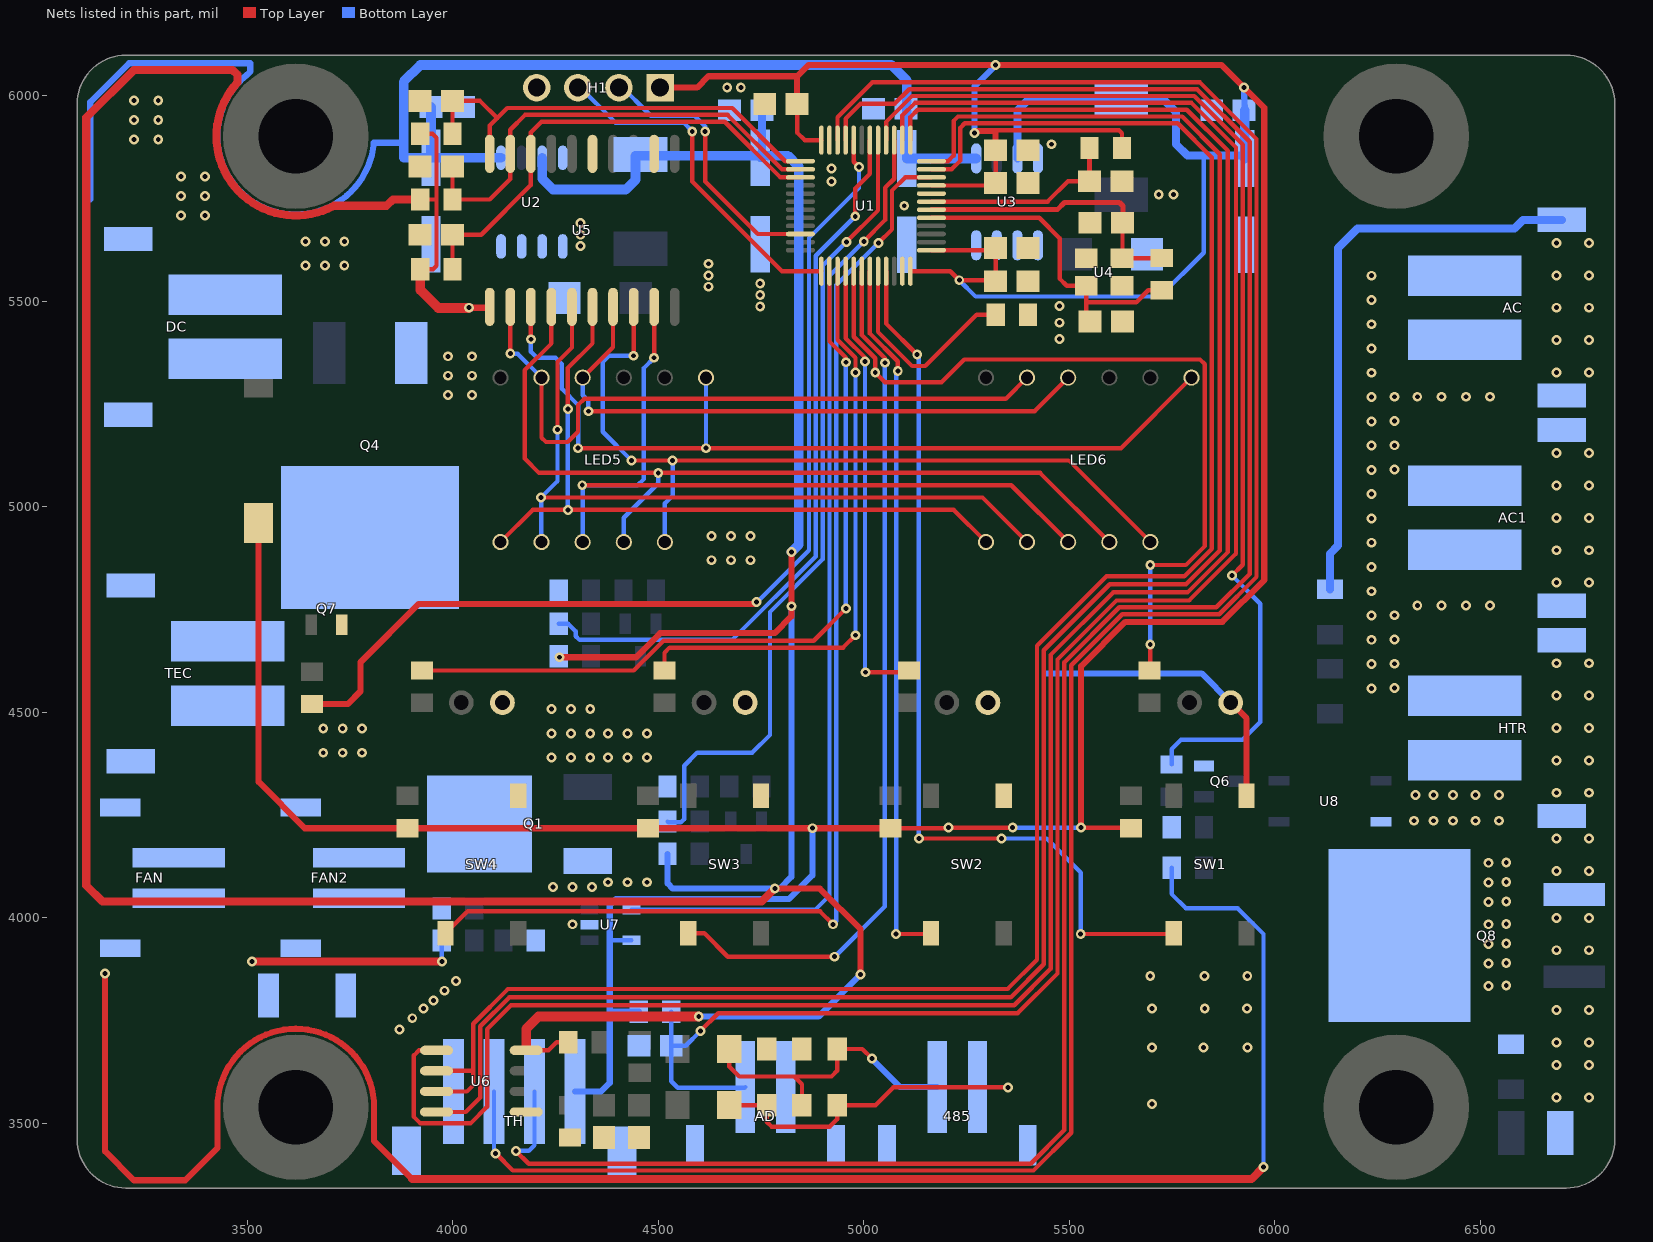
[diagram p0: the nets of this part, all layers, seen from the top]
# Altium PCB MISC82750.pcbdoc (part 2 of 3)
Units mil, origin at the board's own origin, x right, y up, seen from the top; angles counter-clockwise.
Board outline 3740.2 x 2755.9 mil, 2 copper layers (Top Layer, Bottom Layer), stack 62.2 mil thick; 106 components, 84 nets, 362 pads, 334 vias.

## Via types
v1: diameter 24, hole 12, Top Layer to Bottom Layer, 334 vias

## Nets (pads, with @x,y where several pads share a name; then routed paths per layer and width w, separated by ;. In a path a pad name is that pad's centre, name@x,y a point inside that pad or via, vN(x,y) a via of type N, cw(c..) or ccw(c..) an arc to the next point about the centre after c; other vN are vias at no path point) (continued)
+3.3V: BUZZER1.1 C7.2 C8.1 C11.2 C12.2 C13.2 C14.2 C20.2 H1.1 L2.1 R3.2 R7.2 R12.2 R13.2 R14.2 R15.2 TH.1 U1.1 U1.9 U1.24 U1.48 U3.3 U7.5 | length 11081.4
  Top Layer w10.6: C11.2@4837.7,5980 4837.7,5910.3 4856.1,5892 U1.24@4896.8,5892 ; R13.2@5065,4218.1 5204.5,4218.1 v1(5205.8,4219.4) v1(5362.2,4219.4) ; U1.48@5113.3,5573.1 5210.4,5573.1 v1(5232.3,5551.2) 5318.2,5551.2 C13.2@5320.7,5548.7 C14.2@5320.7,5629.4 5315.5,5624.2 U1.1@5164.5,5624.2 ; U1.9@5164.5,5781.7 5314.9,5781.7 C12.2@5320.7,5787.5 C20.2@5320.7,5867.5 ; 5320.7,5913.8 5320.7,5916.1 5620.9,5916.1 5628,5909 R3.2@5628,5873.1 ; v1(5528.5,4219.4) 5648.8,4219.4 R12.2@5650,4218.1
  Top Layer w15: BUZZER1.1@3527.6,4960.6 3527.6,4330.7 3640.1,4218.1 R15.2@3890,4218.1 R14.2@4475,4218.1 v1(4875.1,4218.1) R13.2@5065,4218.1 ; H1.1@4504.3,6019.7 4594.5,6019.7 4622,6047.2 4837.7,6047.2 ; C11.2@4837.7,5980 4837.7,6047.2 ; v1(5269.5,5909.4) 5274,5914 5320.5,5914 5320.7,5913.8 C20.2@5320.7,5867.5 ; v1(5528.5,4219.4) 5528.5,4612.1 5636.3,4720 5872.4,4720 5974.2,4821.7 5974.2,5970.7 v1(5925.2,6019.7) 5870.3,6074.6 v1(5320.7,6074.6) 4865.1,6074.6 4837.7,6047.2
  Bottom Layer w10.6: 4381.9,3945.6 U7.5@4434.9,3945.6 ; v1(5232.3,5551.2) 5272,5511.5 5720.2,5511.5 5826.8,5618.1 5826.8,5854.3 ; v1(5362.2,4219.4) v1(5528.5,4219.4)
  Bottom Layer w15: TH.1@4297.2,3577.6 4361,3577.6 4381.9,3598.4 4381.9,3771.7 ; R7.2@4452.8,3771.7 4381.9,3771.7 ; v1(4875.1,4218.1) 4875.1,4103.5 4817.3,4045.7 4396.9,4045.7 4381.9,4030.7 4381.9,3945.6 4381.9,3771.7 ; v1(5269.5,5909.4) 5269.5,6023.4 v1(5320.7,6074.6) ; v1(5925.2,6019.7) C7.2@5926.6,5964.6
  Bottom Layer w19.7: U3.3@5373.6,5847.4 5373.6,5964.1 5401.6,5992.1 5622.6,5992.1 L2.1@5626,5988.7 5731.8,5988.7 5759.8,5960.6 5759.8,5881.9 5787.4,5854.3 5826.8,5854.3 5919.6,5854.3 C8.1@5926.6,5847.4
  Bottom Layer w23.6: C8.1@5926.6,5847.4 C7.2@5926.6,5964.6
+5V: C3.2 C4.1 L1.1 R4.2 R5.2 R6.2 R20.1 R25.1 R35.2 U2.3 U5.1 U6.8 | length 10482.4
  Top Layer w10.6: R6.2@3920.7,5578.1 3952.1,5578.1 3960.6,5586.6 3960.6,5630.5 3960.4,5630.8 3960.4,5748.3 ; R5.2@3920.7,5747.5 3959.6,5747.5 3960.4,5748.3 ; R4.2@3920.7,5907.5 3950.7,5907.5 3960.6,5897.6 3960.6,5859.1 3960.4,5858.8 3960.4,5748.3 ; U6.8@4178.6,3677.7 4232.8,3677.7 4252.6,3697.5 R35.2@4280.7,3697.5
  Top Layer w15: v1(4039.4,5484.3) 4088,5484.3 U5.1@4090,5486.3 ; v1(4259.8,4633.9) 4445.9,4633.9 4504.9,4692.9 4783.5,4692.9 4824,4733.4 v1(4824,4758) v1(4824,4889.8) ; v1(4783.5,4071.1) 4893.4,4071.1 4992.1,3972.4 v1(4992.1,3862.2)
  Top Layer w19.7: 3475.81,6031.99 ccw(c3618.1,5901.6) 3425.1,5901.6 ccw(c3618.1,5901.6) 3710.78,5732.31 3838.6,5732.3 3854.3,5748 3920.2,5748 R5.2@3920.7,5747.5 ; 3475.9,6032 3475.9,6051.7 3464.6,6063 3224.4,6063 3108.3,5946.9 3108.3,4078.7 3147.6,4039.4 4751.7,4039.4 v1(4783.5,4071.1)
  Top Layer w23.6: R6.2@3920.7,5578.1 3921.3,5577.5 3921.3,5527.6 3965,5483.8 4039,5483.8 v1(4039.4,5484.3) ; U6.8@4178.6,3677.7 4178.6,3729.7 4208.7,3759.8 v1(4598.4,3759.8)
  Bottom Layer w10.6: R25.1@4257.6,4636.6 4257.6,4636.1 v1(4259.8,4633.9)
  Bottom Layer w15: R20.1@4522.6,4155.6 4522.6,4083.7 4535.2,4071.1 v1(4783.5,4071.1) 4795.5,4071.1 4824,4099.5 v1(4824,4758) ; v1(4598.4,3759.8) 4889.8,3759.8 v1(4992.1,3862.2)
  Bottom Layer w19.7: C4.1@4747.8,5849.1 4752,5853.3 4752,5854.3 C3.2@4752,5964.6
  Bottom Layer w23.6: U2.3@4217.6,5849.1 4217.6,5798.1 4244.1,5771.7 4420.9,5771.7 4444.5,5795.3 4444.5,5854.3 4752,5854.3 4815,5854.3 4841.6,5827.7 4841.6,4907.4 v1(4824,4889.8)
A: LED5.11 LED6.11 U5.2 | length 1648.6
  Top Layer w10.6: v1(4140,5372.5) U5.2@4140,5486.3 ; LED5.11@4216.1,5314.2 4216.1,5168.1 4226.8,5157.5 4280,5157.5 4304.8,5182.3 4304.8,5247.3 4320,5262.5 5345.6,5262.5 LED6.11@5397.2,5314.2
  Bottom Layer w10.6: v1(4140,5372.5) 4157.8,5372.5 LED5.11@4216.1,5314.2
AD: AD.1 C19.2 R7.1 U1.14 | length 4591.6
  Top Layer w10.6: v1(4602.4,3724.4) 4645.7,3767.7 5374.2,3767.7 5471.1,3864.6 5471.1,4628.4 5614.7,4772 5791.4,4772 5905.5,4886.1 5905.5,5874.2 5797.1,5982.6 5124.4,5982.6 5093.6,5951.9 U1.14@5093.6,5892
  Bottom Layer w10.6: R7.1@4531.5,3771.7 C19.2@4531.5,3689 ; v1(4602.4,3724.4) 4566.9,3689 C19.2@4531.5,3689 ; AD.1@4711.7,3588.4 4710,3586.6 4547.2,3586.6 4531.5,3602.4 C19.2@4531.5,3689
AD5: U1.15 U7.4 | length 2398.5
  Top Layer w10.6: v1(5000,5645.7) 5051.9,5697.6 5051.9,5776.2 5073.9,5798.2 U1.15@5073.9,5892
  Bottom Layer w10.6: U7.4@4434.9,4020.4 4882.6,4020.4 4916.4,4054.2 4916.4,5562.1 v1(5000,5645.7)
B: LED5.7 LED6.7 U5.3 | length 2152.8
  Top Layer w10.6: v1(4190,5407.5) U5.3@4190,5486.3 ; v1(4305,5142.5) v1(4616.1,5142.5) 5625.6,5142.5 LED6.7@5797.2,5314.2
  Bottom Layer w10.6: v1(4190,5407.5) 4190,5377.5 4205,5362.5 4250,5362.5 4265,5347.5 4265,5287.5 4305,5247.5 v1(4305,5142.5) ; v1(4616.1,5142.5) LED5.7@4616.1,5314.2
BOOT0: R2.2 U1.44 | length 519.9
  Top Layer w10.6: U1.44@5034.6,5573.1 5034.6,5425.4 5117.5,5342.5 5149.6,5342.5 5274.6,5467.5 R2.2@5320.7,5467.5
BUZZER: R38.1 U1.20 | length 2459
  Top Layer w10.6: U1.20@4975.5,5892 4975.5,5839.5 v1(4988.2,5826.8)
  Top Layer w15: R38.1@3657.5,4520.1 3744.5,4520.1 3775.6,4551.2 3775.6,4622 3917.3,4763.8 4734.8,4763.8 v1(4739.1,4768.1)
  Bottom Layer w10.6: v1(4739.1,4768.1) 4740.6,4768.1 4866.6,4894.1 4866.6,5654 4988.2,5775.6 v1(4988.2,5826.8)
C: LED5.4 LED6.4 U5.4 | length 2105.2
  Top Layer w10.6: U5.4@4240,5486.3 4240,5397.5 4175,5332.5 4175,5117.5 4210,5082.5 v1(4500,5082.5) 5428.9,5082.5 LED6.4@5597.2,4914.2
  Bottom Layer w10.6: LED5.4@4416.1,4914.2 4416.1,4973.6 4500,5057.5 v1(4500,5082.5)
CLK: C17.2 R5.1 U1.26 U5.19 | length 1136.5
  Top Layer w10.6: C17.2@3999.4,5827.5 R5.1@3999.4,5747.5 4090,5747.5 4140,5797.5 U5.19@4140,5858.7 4140,5917.5 4175.8,5953.3 4668.7,5953.3 4800.9,5821.1 U1.26@4845.6,5821.1
D: LED5.2 LED6.2 U5.5 | length 1830.7
  Top Layer w10.6: v1(4215,5022.5) 5288.9,5022.5 LED6.2@5397.2,4914.2 ; v1(4255,5187.5) 4255,5352.5 4290,5387.5 U5.5@4290,5486.3
  Bottom Layer w10.6: LED5.2@4216.1,4914.2 4215,4915.3 v1(4215,5022.5) 4255,5062.5 v1(4255,5187.5)
DIN: C18.2 R6.1 U1.27 U5.18 | length 1175
  Top Layer w10.6: R6.1@3999.4,5578.1 C18.2@3999.4,5662 4069.5,5662 4190,5782.5 U5.18@4190,5858.7 4190,5910.6 4216.1,5936.7 4661.8,5936.7 4797.1,5801.4 U1.27@4845.6,5801.4
DP: LED5.3 LED6.3 U5.9 | length 1963.6
  Top Layer w10.6: v1(4315,5052.5) 5358.9,5052.5 LED6.3@5497.2,4914.2 ; v1(4490,5362.5) U5.9@4490,5486.3
  Bottom Layer w10.6: LED5.3@4316.1,4914.2 4316.1,5051.4 v1(4315,5052.5) 4450,5052.5 4465,5067.5 4465,5337.5 v1(4490,5362.5)
E: LED5.1 LED6.1 U5.6 | length 1764.6
  Top Layer w10.6: LED5.1@4116.1,4914.2 4194.5,4992.5 v1(4280,4992.5) 5218.9,4992.5 LED6.1@5297.2,4914.2 ; v1(4280,5237.5) 4280,5337.5 4340,5397.5 U5.6@4340,5486.3
  Bottom Layer w10.6: v1(4280,4992.5) v1(4280,5237.5)
ES485-A: 485.2 D4.1 D5.1 L3.2 | length 856.7
  Top Layer w10.6: L3.2@4672.7,3544.2 D4.1@4763.9,3544.2 4763.9,3503.8 4775.6,3492.1 4917.3,3492.1 4935,3509.8 D5.1@4935,3544.2 5028.5,3544.2 5071.8,3587.5 v1(5350.4,3587.5)
  Bottom Layer w10.6: 485.2@5276.7,3588.4 5349.5,3588.4 v1(5350.4,3587.5)
ES485-B: 485.1 D3.1 D5.2 L4.2 | length 732.6
  Top Layer w10.6: L4.2@4672.7,3680.8 4672.7,3638.3 4696.9,3614.2 4830.7,3614.2 ; D3.1@4849.5,3544.2 4849.5,3595.4 4830.7,3614.2 ; v1(5019.7,3657.5) 4996.3,3680.8 D5.2@4935,3680.8 4935,3628 4921.3,3614.2 4830.7,3614.2
  Bottom Layer w15: v1(5019.7,3657.5) 5088.8,3588.4 485.1@5178.3,3588.4
F: LED5.10 LED6.10 U5.7 | length 1491.2
  Top Layer w10.6: LED5.10@4316.1,5314.2 4390,5388.1 U5.7@4390,5486.3 ; v1(4330,5232.5) 5415.6,5232.5 LED6.10@5497.2,5314.2
  Bottom Layer w10.6: LED5.10@4316.1,5314.2 4316.1,5271.4 4330,5257.5 v1(4330,5232.5)
FAN: R21.1 U1.17 | length 1970.1
  Top Layer w10.6: v1(4958.1,5644.6) 5034.6,5721.1 U1.17@5034.6,5892
  Bottom Layer w10.6: R21.1@4522.6,4234.4 4524.6,4232.3 4555.1,4232.3 4563,4240.2 4563,4370.1 4594.5,4401.6 4728.3,4401.6 4771.7,4444.9 4771.7,4744.1 4899.8,4872.3 4899.8,5586.3 v1(4958.1,5644.6)
FAN1: FAN2.1 FAN2.4 FAN.1 Q1.3
FAN2: FAN2.2 FAN.2 R18.2 R19.1
G: LED5.5 LED6.5 U5.8 | length 2019.5
  Top Layer w10.6: v1(4435,5112.5) v1(4535,5112.5) 5498.9,5112.5 LED6.5@5697.2,4914.2 ; v1(4440,5367.5) U5.8@4440,5486.3
  Bottom Layer w10.6: v1(4435,5112.5) 4365,5182.5 4365,5352.5 4380,5367.5 v1(4440,5367.5) ; LED5.5@4516.1,4914.2 4516.1,5008.6 4535,5027.5 v1(4535,5112.5)
GND: 485.3 485.4 AD.2 AD.3 AD.4 C1.2 C2.2 C3.1 C4.2 C5.2 C6.2 C7.1 C8.2 C9.1 C10.1 C11.1 C12.1 C13.1 C14.1 C15.1 C16.1 C17.1 C18.1 C19.1 C20.1 C21.1 C22.1 D1.2 D2.2 D3.2 D4.2 DC.2 H1.4 LED1.2 LED2.2 LED3.2 LED4.2 Q1.2 Q4.3 Q6.2 Q7.2 R2.1 R16.2 R23.1 R27.1 R29.2 R37.1 SW1.4 SW2.4 SW3.4 SW4.4 TH.4 TH.5 TH.6 U1.8 U1.23 U1.47 U2.4 U2.5 U2.6 U2.7 U2.8 U3.4 U3.5 U3.6 U3.7 U3.8 U4.2 U4.4 U5.12 U5.15 U6.5 U7.2 | length 723.4
  Top Layer w15: LED4.2@5892.5,4523.6 5931.1,4485 SW1.4@5931.1,4297.2
  Bottom Layer w15: 5440.9,4594.5 5821.7,4594.5 LED4.2@5892.5,4523.6
  other v1: 5700.8,3547.2 5700.8,3685 5826.5,3685 5933.1,3685 3870.1,3728.3 3901.6,3755.9 3929.1,3779.5 5700.8,3779.5 5829.5,3779.5 5932,3779.5 3952.8,3799.2 3980.3,3822.8 4007.9,3846.5 5696.9,3858.3 5828.5,3858.3 5933,3858.3 4291.3,3984.3 4244.1,4074.8 4291.3,4074.8 4338.6,4074.8 4378,4086.6 4425.2,4086.6 4472.4,4086.6 4240.2,4389.8 4287.4,4389.8 4334.6,4389.8 4378,4389.8 4425.2,4389.8 4472.4,4389.8 3685,4401.6 3732.3,4401.6 3779.5,4401.6 4240.2,4448.8 4287.4,4448.8 4334.6,4448.8 4378,4448.8 4425.2,4448.8 4472.4,4448.8 3685,4460.6 3732.3,4460.6 3779.5,4460.6 4240.2,4507.9 4287.4,4507.9 4334.6,4507.9 4629.9,4870.1 4677.2,4870.1 4724.4,4870.1 4629.9,4929.1 4677.2,4929.1 4724.4,4929.1 3988.2,5271.7 4047.2,5271.7 3988.2,5318.9 4047.2,5318.9 3988.2,5366.1 4047.2,5366.1 5475.9,5407.8 5475.9,5447.8 4748,5487.5 5475.9,5488.2 4748,5515 4622,5535.4 4748,5543.3 4622,5562.9 3641.7,5586.6 3689,5586.6 3736.2,5586.6 4622,5591.2 4310.9,5634.2 3641.7,5645.7 3689,5645.7 3736.2,5645.7 4310.9,5661.7 4310.9,5690 3338.6,5708.7 3397.6,5708.7 5098.4,5732.3 3338.6,5755.9 3397.6,5755.9 5717.5,5759.6 5753.6,5759.6 4921.3,5791.3 3338.6,5803.1 3397.6,5803.1 4921.3,5822.8 5456.7,5881.9 3224.4,5893.7 3283.5,5893.7 3224.4,5940.9 3283.5,5940.9 3224.4,5988.2 3283.5,5988.2 4667.7,6019.7 4700.8,6019.7
HTR: R28.1 U1.16 | length 2711.5
  Top Layer w10.6: U1.16@5054.2,5892 5054.2,5936 5117.5,5999.3 5804,5999.3 5922.1,5881.1 5922.1,4859.1 v1(5895.8,4832.8)
  Bottom Layer w10.6: R28.1@5748.8,4373.2 5748.8,4410.3 5771.7,4433.1 5921.3,4433.1 5964.6,4476.4 5964.6,4764.1 v1(5895.8,4832.8)
HTR1: HTR.2 Q8.2 R33.2 U8.4
  other v1: 6519.7,3834.6 6563,3835.3 6519.7,3889.1 6563,3889.8 6519.7,3936.7 6563,3937.4 6519.7,3984.3 6563,3984.9 6519.7,4038.7 6563,4039.4 6519.7,4086.3 6563,4087 6519.7,4133.9 6563,4134.5 6338.6,4236.2 6386.1,4236.2 6433.7,4236.2 6488.2,4236.2 6545.5,4236.2 6342.5,4299.2 6385.5,4299.2 6433.7,4299.2 6488.2,4299.2 6545.5,4299.2
K1: SW4.1 U1.10 | length 2931.6
  Top Layer w10.6: SW4.1@3982.3,3962.6 4035.4,4015.7 4893.7,4015.7 v1(4925.2,3984.3) ; v1(5035.4,5641.7) 5068.5,5674.8 5068.5,5769.3 5100.6,5801.4 U1.10@5164.5,5801.4
  Bottom Layer w10.6: v1(4925.2,3984.3) 4933.1,3992.1 4933.1,5539.4 v1(5035.4,5641.7)
K2: SW3.1 U1.42 | length 2121.3
  Top Layer w10.6: SW3.1@4572.8,3962.6 4612.2,3962.6 4669.3,3905.5 v1(4929.1,3905.5) ; U1.42@4995.2,5573.1 4995.2,5417.8 5051.2,5361.8 v1(5051.2,5350.4)
  Bottom Layer w10.6: v1(4929.1,3905.5) 5051.2,4027.6 v1(5051.2,5350.4)
K3: SW2.1 U1.43 | length 1727.8
  Top Layer w10.6: U1.43@5014.9,5573.1 5014.9,5421.6 5082.7,5353.8 v1(5082.7,5330.7) ; v1(5078.7,3960.6) 5161.4,3960.6 SW2.1@5163.4,3962.6
  Bottom Layer w10.6: v1(5078.7,3960.6) 5078.7,5326.8 v1(5082.7,5330.7)
K4: SW1.1 U1.45 | length 2217.9
  Top Layer w10.6: U1.45@5054.2,5573.1 5054.2,5445.8 v1(5129.9,5370.1) ; v1(5133.9,4192.9) v1(5334.6,4192.9) ; v1(5527.7,3960.6) 5752,3960.6 SW1.1@5753.9,3962.6
  Bottom Layer w10.6: v1(5129.9,5370.1) 5133.9,5366.1 v1(5133.9,4192.9) ; v1(5334.6,4192.9) 5444.9,4192.9 5527.7,4110.1 v1(5527.7,3960.6)
L: AC1.1 AC.1 HTR.1
  other v1: 6235.5,4558.3 6291.3,4559.1 6235.5,4617.3 6291.3,4618.1 6235.5,4676.4 6291.3,4677.2 6235.5,4735.4 6291.3,4736.2 6346.5,4759.8 6405.5,4759.8 6464.6,4759.8 6523.6,4759.8 6235.5,4794.5 6235.5,4853.5 6235.5,4912.6 6235.5,4971.7 6235.5,5030.7 6235.5,5089.8 6291.3,5090.6 6235.5,5148.8 6291.3,5149.6 6235.5,5207.9 6291.3,5208.7 6235.5,5266.9 6291.3,5267.7 6346.5,5267.7 6405.5,5267.7 6464.6,5267.7 6523.6,5267.7 6235.5,5326 6235.5,5385 6235.5,5444.1 6235.5,5503.2 6235.5,5562.2
LED1: R8.2 U1.38 | length 1930.9
  Top Layer w10.6: R8.2@3925,4601.9 4440.5,4601.9 4512.7,4674.1 4878,4674.1 v1(4956.4,4752.5) ; U1.38@4916.5,5573.1 4916.5,5402.4 4956.4,5362.5 v1(4956.4,5351.6)
  Bottom Layer w10.6: v1(4956.4,4752.5) v1(4956.4,5351.6)
LED2: R9.2 U1.39 | length 1429
  Top Layer w10.6: R9.2@4515,4601.9 4515,4645 4527.6,4657.5 4949.7,4657.5 v1(4979.7,4687.5) ; U1.39@4936.1,5573.1 4936.1,5406.3 4979.7,5362.7 v1(4979.7,5326.8)
  Bottom Layer w10.6: v1(4979.7,4687.5) v1(4979.7,5326.8)
LED3: R10.2 U1.40 | length 1103.5
  Top Layer w10.6: U1.40@4955.8,5573.1 4955.8,5410.1 5003,5362.9 v1(5003,5353.4) ; v1(5003.9,4597.5) 5105.7,4597.5 R10.2@5110,4601.9
  Bottom Layer w10.6: v1(5003,5353.4) 5003,4598.4 v1(5003.9,4597.5)
LED4: R11.2 U1.41 | length 1958.8
  Top Layer w10.6: U1.41@4975.5,5573.1 4975.5,5413.9 5027.9,5361.6 v1(5027.9,5326.8) 5051.5,5303.1 5189,5303.1 5244.1,5358.3 5818,5358.3 5829.8,5346.5 5829.8,4904.5 5783.6,4858.3 v1(5696.9,4858.3) ; R11.2@5695,4601.9 5696.9,4603.7 v1(5696.9,4665.4)
  Bottom Layer w10.6: v1(5696.9,4665.4) v1(5696.9,4858.3)
N: AC1.2 AC1.3 AC1.4 AC.2 AC.3 AC.4 C23.1 HTR.3 HTR.4 Q8.1 R32.2 | length 1411.6
  Bottom Layer w19.7: R32.2@6133.9,4799.2 6133.9,4885.8 6153.5,4905.5 6153.5,5629.9 6200.8,5677.2 6582.7,5677.2 6603.5,5698 AC.4@6698.1,5698
  other v1: 6685,3563 6763.8,3563 6685,3641.7 6763.8,3641.7 6685,3696.9 6763.8,3696.9 6685,3775.6 6763.8,3775.6 6685,3921.3 6763.8,3921.3 6685,4000 6763.8,4000 6685,4114.2 6763.8,4114.2 6685,4192.9 6763.8,4192.9 6685,4304.3 6763.8,4304.3 6685,4383.1 6763.8,4383.1 6685,4461.8 6763.8,4461.8 6685,4540.6 6763.8,4540.6 6685,4619.3 6763.8,4619.3 6685,4815.6 6763.8,4815.6 6685,4894.3 6763.8,4894.3 6685,4973 6763.8,4973 6685,5051.8 6763.8,5051.8 6685,5130.5 6763.8,5130.5 6685,5326.8 6763.8,5326.8 6685,5405.5 6763.8,5405.5 6685,5484.3 6763.8,5484.3 6685,5563 6763.8,5563 6685,5641.7 6763.8,5641.7
NRST: C15.2 R3.1 U1.7 | length 486.4
  Top Layer w10.6: U1.7@5164.5,5742.4 5447.1,5742.4 5496.6,5791.9 C15.2@5549.2,5791.9
  Top Layer w12.1: C15.2@5549.2,5791.9 R3.1@5549.2,5873.1
OSCIN: C9.2 R1.2 U1.5 U4.3 | length 789
  Top Layer w10.6: U1.5@5164.5,5703 5426.9,5703 5476.4,5653.5 5476.4,5555.1 5493.9,5537.6 U4.3@5541.5,5537.6 5541.5,5497.2 ; C9.2@5550.4,5451 5541.5,5460 5541.5,5497.2 ; R1.2@5724.8,5526.7 5692,5526.7 5662.6,5497.2 5541.5,5497.2
OSCOUT: C10.2 R1.1 U1.6 U4.1 | length 702.1
  Top Layer w10.6: C10.2@5629.2,5691 5629.2,5605.5 U4.1@5628.1,5604.5 5723.9,5604.5 R1.1@5724.8,5605.4
  Top Layer w12.1: U1.6@5164.5,5722.7 5470.7,5722.7 5488.2,5740.2 5622,5740.2 5630.6,5731.6 5630.6,5692.5 C10.2@5629.2,5691
P: R24.1 U1.18 | length 1799.5
  Top Layer w10.6: v1(4979.2,5706.7) 4979.2,5774.4 5014.9,5810.2 U1.18@5014.9,5892
  Bottom Layer w10.6: R24.1@4257.6,4715.3 4280.7,4715.3 4299.2,4696.9 4299.2,4685 4307.1,4677.2 4309.1,4677.2 4309.3,4676.9 4680.8,4676.9 4883.2,4879.2 4883.2,5610.7 v1(4979.2,5706.7)
PL: Q4.4 TEC.2
RD: U1.11 U6.2 U6.3 | length 4820
  Top Layer w10.6: U6.3@3960.6,3577.7 4034.4,3577.7 4050.3,3593.6 4050.3,3627.7 4047.2,3627.7 ; U6.2@3960.6,3627.7 4047.2,3627.7 ; U1.11@5164.5,5821.1 5213.6,5821.1 5235,5842.5 5235,5922.1 5245.7,5932.8 5763.5,5932.8 5846.5,5849.8 5846.5,4897.6 5779.9,4831.1 5590.3,4831.1 5421.3,4662 5421.3,3898.3 5349.8,3826.8 4134.1,3826.8 4049.9,3742.6 4049.9,3630.4 4047.2,3627.7
RXD: U1.13 U6.1 | length 5184
  Top Layer w10.6: U6.1@3960.6,3677.7 3917.9,3677.7 3905.5,3665.4 3905.5,3515.7 3921.3,3500 4043.3,3500 4083.6,3540.3 4083.6,3729.2 4141.7,3787.4 5366.1,3787.4 5454.5,3875.9 5454.5,4639.6 5606.6,4791.7 5787.6,4791.7 5885.8,4890 5885.8,5866.1 5785.9,5966 5131.3,5966 5113.3,5948.1 U1.13@5113.3,5892
SCL: TH.3 U1.22 | length 5517.7
  Top Layer w10.6: v1(4104.4,3427.1) 4146.2,3385.3 5412.8,3385.3 5504.4,3477 5504.4,4614.6 5628.5,4738.8 5864.6,4738.8 5955.4,4829.5 5955.4,5894.9 5817.8,6032.5 5020.8,6032.5 4936.1,5947.8 U1.22@4936.1,5892
  Bottom Layer w10.6: TH.3@4100.4,3577.6 4100.4,3431.1 v1(4104.4,3427.1)
SDA: TH.2 U1.21 | length 5409.8
  Top Layer w10.6: v1(4153.5,3433.1) 4184.7,3402 5405.9,3402 5487.8,3483.8 5487.8,4621.5 5621.6,4755.4 5857.7,4755.4 5938.8,4836.4 5938.8,5888 5810.9,6015.9 5110.6,6015.9 5075,5980.3 4992.1,5980.3 4955.8,5944 U1.21@4955.8,5892
  Bottom Layer w10.6: v1(4153.5,3433.1) 4185,3433.1 4198.8,3446.9 TH.2@4198.8,3577.6
STB: C16.2 R4.1 U1.25 U5.20 | length 1101.6
  Top Layer w10.6: R4.1@3999.4,5907.5 C16.2@3999.4,5987.5 4066.3,5987.5 4108.1,5945.6 ; U5.20@4090,5858.7 4090,5927.5 4108.1,5945.6 ; U1.25@4845.6,5840.8 4808.8,5840.8 4679.7,5970 4132.5,5970 4108.1,5945.6
SWCLK: H1.3 U1.37 | length 868.7
  Top Layer w10.6: v1(4582.7,5913.4) 4582.7,5791.3 4800.9,5573.1 U1.37@4896.8,5573.1
  Bottom Layer w10.6: H1.3@4304.3,6043.3 4304.3,6026.4 4396.1,5934.6 4561.4,5934.6 v1(4582.7,5913.4)
SWDIO: H1.2 U1.34 | length 685.5
  Top Layer w10.6: v1(4614.2,5913.4) 4614.2,5791.3 4741.9,5663.6 U1.34@4845.6,5663.6
  Bottom Layer w10.6: H1.2@4404.3,6043.3 4404.3,6028.7 4481.8,5951.3 4588.1,5951.3 4614.2,5925.2 v1(4614.2,5913.4)
TXD: U1.12 U6.4 | length 4818.3
  Top Layer w10.6: U6.4@3960.6,3527.7 3960.8,3527.6 4031.5,3527.6 4066.9,3563 4066.9,3736.1 4137.9,3807.1 5357.9,3807.1 5437.9,3887.1 5437.9,4650.8 5598.4,4811.4 5783.7,4811.4 5866.1,4893.8 5866.1,5857.9 5774.7,5949.4 5229,5949.4 5218.4,5938.8 5218.4,5854.3 5204.9,5840.8 U1.12@5164.5,5840.8
VCC: C1.1 C2.1 C5.1 C6.1 DC.1 DC.3 DC.4 FAN2.3 FAN.3 FAN.4 R17.2 R19.2 R30.2 TEC.1 TEC.3 TEC.4 U2.1 U3.1 | length 8853.8
  Top Layer w15: v1(3154.3,3864.3) 3154.3,3431.9 3224.4,3361.8 3349.4,3361.8 3427.5,3439.9 3427.5,3539.4 cw(c3618.1,3539.4) 3808.7,3539.4 3808.7,3457 3901.6,3364.2
  Top Layer w19.7: v1(3511.8,3893.7) v1(3973.6,3893.7) ; 3901.6,3364.2 5942.9,3364.2 v1(5972.4,3393.7)
  Bottom Layer w10.6: v1(3973.6,3893.7) R17.2@3973.6,3944.9 ; R30.2@5748.8,4122 5748.8,4058.2 5783.5,4023.6 5909.4,4023.6 5972.4,3960.6 v1(5972.4,3393.7)
  Bottom Layer w15: 3118.1,5748 3118.1,5984.5 3212.7,6079.1 3507.5,6079.1 3507.5,6058.7 3500.1,6051.3 ; 3500.23,6051.38 ccw(c3618.1,5901.6) 3427.5,5901.6 ccw(c3618.1,5901.6) 3427.84,5890.3 ccw(c3618.1,5901.6) 3432.69,5857.43 ccw(c3618.1,5901.6) 3808.03,5885.65 ; 3808.1,5885.5 3880.6,5885.5
  Bottom Layer w23.6: C2.1@3947.2,5972.4 C1.1@3947.2,5849.1 ; U2.1@4117.6,5849.1 C1.1@3947.2,5849.1 ; U3.1@5273.6,5847.4 C5.1@5104.6,5847.4 5104.6,6037.1 5066.9,6074.8 3921.3,6074.8 3880.6,6034.1 3880.6,5885.5 3880.6,5849.1 C1.1@3947.2,5849.1
pads on no net: SW1.3 SW2.3 SW3.3 SW4.3 U1.2 U1.3 U1.4 U1.19 U1.28 U1.29 U1.30 U1.31 U1.32 U1.33 U1.35 U1.36 U1.46
copper on no net:
  other v1: 3589.6,3414.4 3642.9,3413.6 6266.7,3414.4 6320,3413.6 3691.9,3434.6 6369,3434.6 3541.2,3436.8 6218.4,3436.8 3728.1,3473.6 6405.3,3473.6 3506.2,3477 6183.3,3477 3745.4,3524.1 6422.5,3524.1 3490.5,3527.9 6167.6,3527.9 3740.6,3577.1 6417.7,3577.1 3496.8,3580.8 6174,3580.8 3714.6,3623.7 6391.8,3623.7 3524.2,3626.6 6201.3,3626.6 3672,3655.7 6349.2,3655.7 3567.7,3657.2 6244.9,3657.2 3620,3667.5 6297.2,3667.5 3642.9,5775.8 6320,5775.8 3589.6,5776.6 6266.7,5776.6 3691.9,5796.8 6369,5796.8 3541.2,5799 6218.4,5799 3728.1,5835.8 6405.3,5835.8 3506.2,5839.2 6183.3,5839.2 3745.4,5886.3 6422.5,5886.3 3490.5,5890.1 6167.6,5890.1 3740.6,5939.3 6417.7,5939.3 3496.8,5943 6174,5943 3714.6,5985.9 6391.8,5985.9 3524.2,5988.8 6201.3,5988.8 3672,6017.9 6349.2,6017.9 3567.7,6019.4 6244.9,6019.4 3620,6029.7 6297.2,6029.7

## Polygon pours and split planes (outlines as drawn)
GND on Top Layer (solid, remove dead copper, pour order 2): 3000,6133.9 3000,3000 5984.3,3000 5984.3,6133.9
VCC on Bottom Layer (solid, remove dead copper, pour order 34): 3094.5,5775.6 3263.8,5775.6 3283.5,5755.9 3283.5,5437 3299.2,5421.3 3586.6,5421.3 3602.4,5405.5 3602.4,5295.3 3515.7,5208.7 3515.7,4811 3472.2,4767.5 3310.8,4767.5 3279.5,4736.2 3279.5,4618.1 3311,4586.6 3590.6,4586.6 3610.2,4566.9 3610.2,4452.8 3590.6,4433.1 3363.6,4433.1 3341,4410.4 3341,4254.4 3322.8,4236.2 3216.5,4236.2 3204.7,4224.4 3204.7,3980.3 3216.5,3968.5 3681.1,3968.5 3696.9,3952.8 3696.9,3901.6 3622,3826.8 3622,3763.8 3606.3,3748 3444.9,3748 3409.4,3712.6 3409.4,3370.1 3393.7,3354.3 3090.6,3354.3 3090.6,5771.7
PL on Bottom Layer (solid, remove dead copper, pour order 36): 3536.6,5126 4011.8,5126 4035.4,5102.4 4035.4,4618.1 4023.6,4606.3 3318.9,4606.3 3303.1,4622 3303.1,4732.3 3316.2,4745.3 3485.5,4745.3 3536.1,4796
FAN1 on Bottom Layer (solid, remove dead copper, pour order 38): 3220.5,4109.8 3220.5,4204.7 3236.2,4220.5 3331.2,4220.5 3358.3,4247.5 3358.3,4330.7 3385.8,4358.3 4192.1,4358.3 4204.7,4345.7 4204.7,4110.2 4192,4097.6 3232.7,4097.6
FAN2 on Bottom Layer (solid, remove dead copper, pour order 40): 3220.5,4070.9 3228.3,4078.7 4000,4078.7 4013,4065.8 4013,3997.6 3999.6,3984.3 3933.1,3984.3 3921.3,3972.4 3921.3,3874 3796.1,3748.9 3717.6,3748.9 3709.8,3756.6 3709.8,3964.7 3690.3,3984.3 3232.3,3984.3 3220.5,3996.1
GND on Bottom Layer (solid, remove dead copper, pour order 42): 3015.7,6129.9 3015.7,3271.3 6003.9,3271.3 6003.9,6129.9
N on Bottom Layer (solid, remove dead copper, pour order 46): 6629.9,5712.6 6649.6,5732.3 6870.1,5732.3 6870.1,3401.2 6629.9,3401.2 6629.9,4818.9 6618.1,4830.7 6322.8,4830.7 6315,4838.6 6315,4944.9 6326.8,4956.7 6618.1,4956.7 6629.9,4968.5 6629.9,5334.6 6622,5342.5 6318.9,5342.5 6311,5350.4 6311,5460.6 6315,5464.6 6622,5464.6 6629.9,5472.4
L on Bottom Layer (solid, remove dead copper, pour order 52): 6610.2,5614.2 6610.2,5503.9 6598.4,5492.1 6315,5492.1 6299.2,5476.4 6299.2,5334.6 6322.8,5311 6590.6,5311 6610.2,5291.3 6610.2,4992.1 6594.5,4976.4 6311,4976.4 6299.2,4964.6 6299.2,4815 6315,4799.2 6594.5,4799.2 6610.2,4783.5 6610.2,4492.1 6598.4,4480.3 6192.9,4480.3 6181.1,4492.1 6181.1,5602.4 6208.7,5629.9 6594.5,5629.9
N on Top Layer (solid, remove dead copper, pour order 4): 6629.9,5712.6 6649.6,5732.3 6854.3,5732.3 6854.3,3401.2 6629.9,3401.2 6629.9,4818.9 6618.1,4830.7 6322.8,4830.7 6315,4838.6 6315,4944.9 6326.8,4956.7 6618.1,4956.7 6629.9,4968.5 6629.9,5334.6 6622,5342.5 6318.9,5342.5 6311,5350.4 6311,5460.6 6315,5464.6 6622,5464.6 6629.9,5472.4
L on Top Layer (solid, remove dead copper, pour order 42): 6610.2,5614.2 6610.2,5503.9 6598.4,5492.1 6315,5492.1 6299.2,5476.4 6299.2,5334.6 6322.8,5311 6590.6,5311 6610.2,5291.3 6610.2,4992.1 6594.5,4976.4 6311,4976.4 6299.2,4964.6 6299.2,4815 6315,4799.2 6594.5,4799.2 6610.2,4783.5 6610.2,4492.1 6598.4,4480.3 6192.9,4480.3 6181.1,4492.1 6181.1,5602.4 6208.7,5629.9 6594.5,5629.9
HTR1 on Top Layer (solid, remove dead copper, pour order 46): 6129.1,3748 6121.2,3755.9 6121.2,4252 6298.3,4429.1 6577.9,4429.1 6577.9,3748
HTR1 on Bottom Layer (solid, remove dead copper, pour order 48): 6129.9,3732.3 6114.2,3748 6114.2,4185 6208.7,4279.5 6291.3,4279.5 6303.1,4291.3 6303.1,4429.1 6322.8,4448.8 6594.5,4448.8 6617.8,4425.5 6617.8,3663.7 6533.8,3664 6465.6,3732.3

## Keep-outs
Board Outline Layer:
  lines w10: 3086.6,5980.3 cw(c3204.7,5980.3) 3204.7,6098.4 6708.7,6098.4 ; 3086.6,5980.3 3086.6,5980.3 ; 3086.6,5980.3 3086.6,3460.6 ccw(c3204.7,3460.6) 3204.7,3342.5 6708.7,3342.5 ; 6708.7,3342.5 6708.7,3342.5 ; 6708.7,3342.5 ccw(c6708.7,3460.6) 6826.8,3460.6 ; 6708.7,6098.4 cw(c6708.7,5980.3) 6826.8,5980.3 ; 6708.7,6098.4 6708.7,6098.4 ; 6826.8,3460.6 6826.8,3460.6 ; 6826.8,3460.6 6826.8,5980.3 ; 6826.8,5980.3 6826.8,5980.3

## Silkscreen, mask and mechanical layers (free items; w line width, h text height)
Top Silkscreen Layer:
  text "ENMG  26B05" at 3334.6,3775.6 h120 r90
Top Solder Mask Layer:
  region: 6598.4,5610.2 6598.4,5519.7 6586.6,5507.9 6307.1,5507.9 6283.5,5484.3 6283.5,5330.7 6318.9,5295.3 6586.6,5295.3 6598.4,5283.5 6598.4,5000 6590.6,4992.1 6311,4992.1 6283.5,4964.6 6283.5,4807.1 6303.1,4787.4 6586.6,4787.4 6598.4,4775.6 6598.4,4500 6590.6,4492.1 6196.9,4492.1 6190.6,4498.4 6190.6,5598.3 6212.6,5620.3 6588.3,5620.3
  region: 6651.2,5718.1 6792.2,5718.1 6803.1,5707.2 6803.1,3889.8 6795.3,3881.9 6655.5,3881.9 6645.7,3891.7 6645.7,4822.8 6626,4842.5 6342.5,4842.5 6330.7,4854.3 6330.7,4929.1 6342.5,4940.9 6626,4940.9 6645.7,4960.6 6645.7,5338.6 6629.9,5354.3 6330.7,5354.3 6322.8,5362.2 6322.8,5444.9 6330.7,5452.8 6626,5452.8 6641.7,5468.5 6641.7,5708.7
  region: 6563,4405.5 6563,3775.6 6551.2,3763.8 6145.7,3763.8 6133.9,3775.6 6133.9,4244.1 6303.9,4414.1 6554.4,4414.1